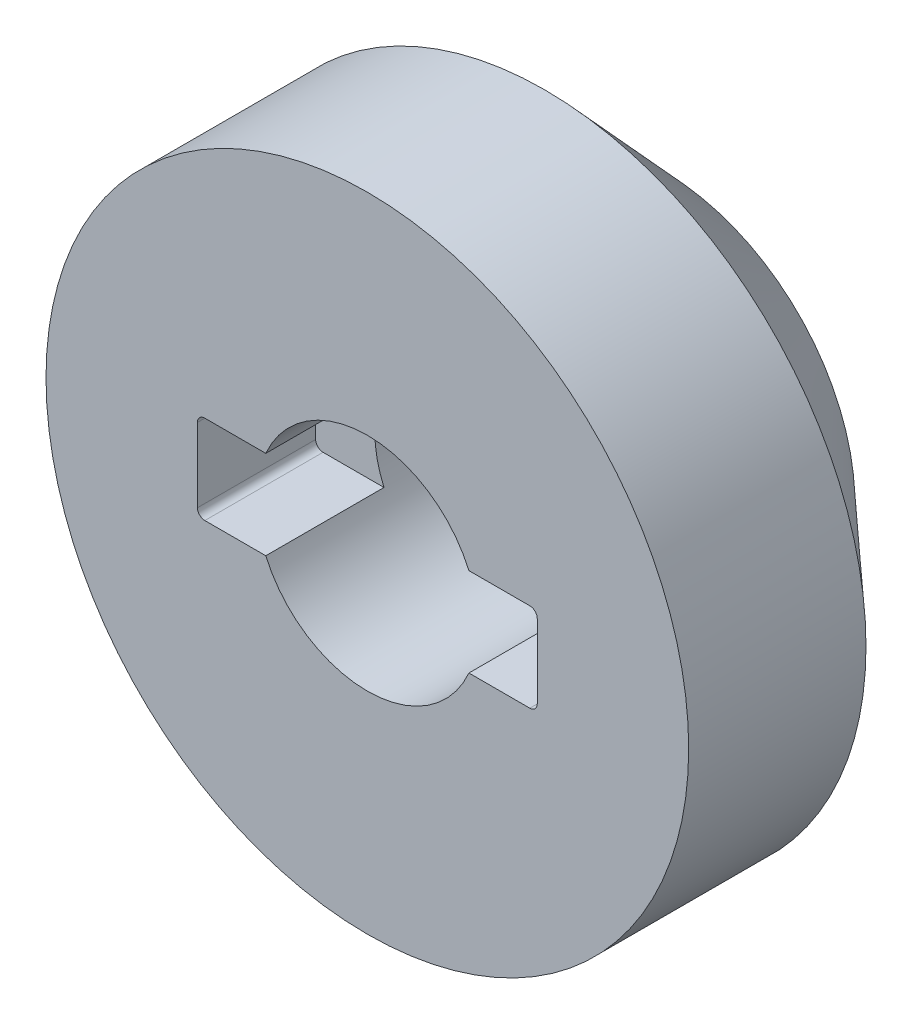
SolidWorks part; units mm, degrees
ref_plane "前视基准面" through (0, 0, 0) normal (0, 0, 1) x (1, 0, 0)
ref_plane "上视基准面" through (0, 0, 0) normal (0, 1, 0) x (1, 0, 0)
ref_plane "右视基准面" through (0, 0, 0) normal (1, 0, 0) x (0, 0, -1)
sketch "草图1" plane through (0, 0, 0) normal (0, 0, 1) x (1, 0, 0)
  circle A0 centre (0, 0) radius 21.75
  circle A1 centre (0, 0) radius 7.5
  dimension "D1" = 43.5
  dimension "D2" = 15
extrude "凸台-拉伸1" add sketch "草图1" along normal blind 12
sketch "草图2" plane through (0, 0, 12) normal (0, 0, 1) x (1, 0, 0)
  line L1 (-11, 3) -> (11, 3)
  line L2 (-11.5, 2.5) -> (-11.5, -2.5)
  line L3 (-11, -3) -> (11, -3)
  line L4 (11.5, 2.5) -> (11.5, -2.5)
  line L5 (-11.5, 3) -> (11.5, -3) construction
  line L6 (-11.5, -3) -> (11.5, 3) construction
  arc A0 (11, 3) -> (11.5, 2.5) centre (11, 2.5) cw
  arc A1 (11, -3) -> (11.5, -2.5) centre (11, -2.5) ccw
  arc A2 (-11.5, -2.5) -> (-11, -3) centre (-11, -2.5) ccw
  arc A3 (-11, 3) -> (-11.5, 2.5) centre (-11, 2.5) ccw
  point P0 (0, 0)
  dimension "D3" = 0.5
  dimension "D1" = 23
  dimension "D2" = 6
extrude "切除-拉伸1" cut sketch "草图2" against normal blind 8
sketch "草图4" plane through (0, 0, 0) normal (0, 0, -1) x (-1, 0, 0)
  circle A0 centre (0, 0) radius 21.75
ref_plane "基准面1" through (0, 0, -8) normal (0, 0, -1) x (-1, 0, 0)
sketch "草图5" plane through (0, 0, -8) normal (0, 0, -1) x (-1, 0, 0)
  circle A0 centre (0, 0) radius 13
  dimension "D1" = 26
loft "放样2" add profiles "草图4", "草图5"
sketch "草图6" plane through (0, 0, 0) normal (0, 0, 1) x (1, 0, 0)
  circle A0 centre (0, 0) radius 6.5
extrude "切除-拉伸3" cut sketch "草图6" against normal blind 48
